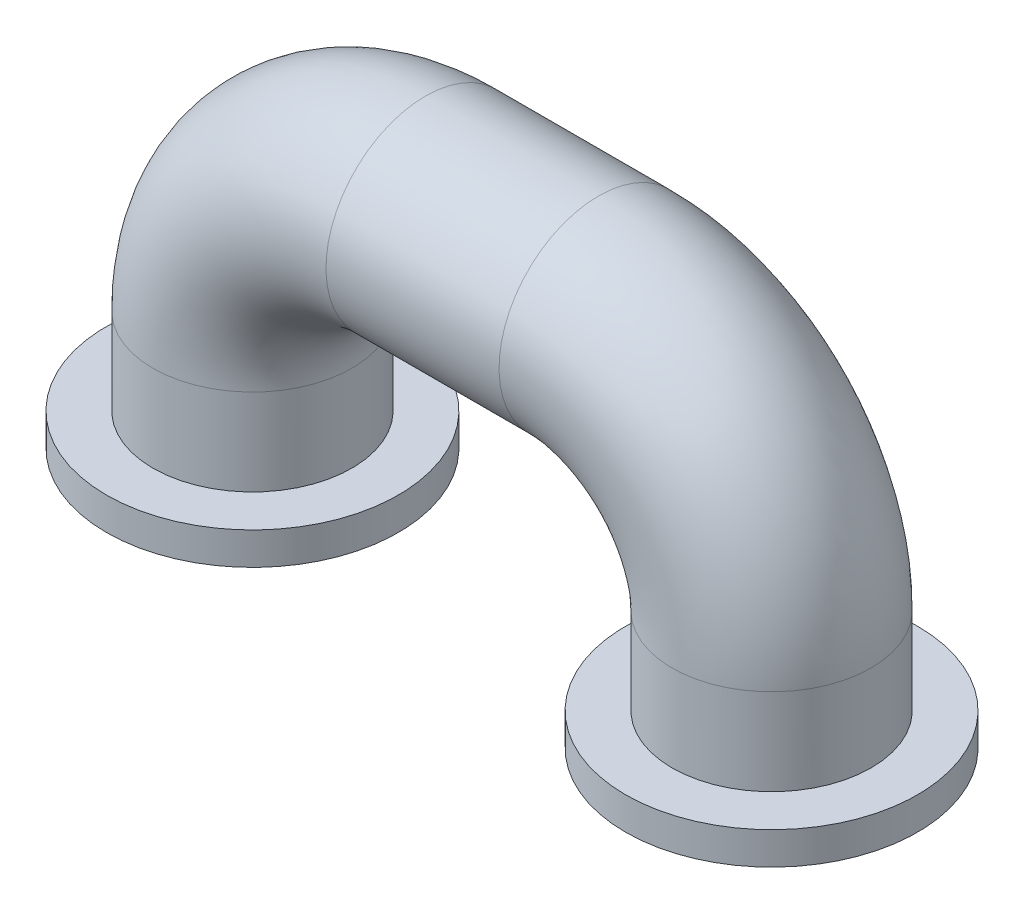
SolidWorks part; units mm, degrees
material "普通碳钢"
ref_plane "Front Plane" through (0, 0, 0) normal (0, 0, 1) x (1, 0, 0)
ref_plane "Top Plane" through (0, 0, 0) normal (0, 1, 0) x (1, 0, 0)
ref_plane "Right Plane" through (0, 0, 0) normal (1, 0, 0) x (0, 0, -1)
sketch "Sketch2" plane through (0, 0, 0) normal (0, 1, 0) x (1, 0, 0)
  circle A0 centre (0, 0) radius 46
  circle A1 centre (0, 0) radius 40
  dimension "D1" = 80
  dimension "D2" = 92
sketch "Sketch3" plane through (0, 0, 0) normal (0, 0, 1) x (1, 0, 0)
  line L0 (0, 0) -> (0, 40)
  line L1 (80, 120) -> (160, 120)
  line L2 (240, 40) -> (240, 0)
  arc A0 (160, 120) -> (240, 40) centre (160, 40) cw
  arc A1 (0, 40) -> (80, 120) centre (80, 40) cw
  point P7 (240, 120)
  point P10 (0, 120)
  dimension "D4" = 80
  dimension "D1" = 120
  dimension "D2" = 240
  dimension "D3" = 120
sweep "Sweep1" add profiles "Sketch2" path "Sketch3"
sketch "Sketch4" plane through (0, 0, 0) normal (0, -1, 0) x (-1, 0, 0)
  circle A0 centre (0, 0) radius 67.5
  circle A1 centre (0, 0) radius 40
  circle A2 centre (-240, 0) radius 40
  circle A3 centre (-240, 0) radius 67.5
  dimension "D1" = 135
  dimension "D2" = 135
extrude "Boss-Extrude1" add sketch "Sketch4" along normal blind 15
sketch "Sketch5" plane through (0, -15, 0) normal (0, -1, 0) x (-1, 0, 0)
  line L0 (0, 0) -> (0, -67.5) construction
  circle A0 centre (0, 0) radius 67.5 construction
